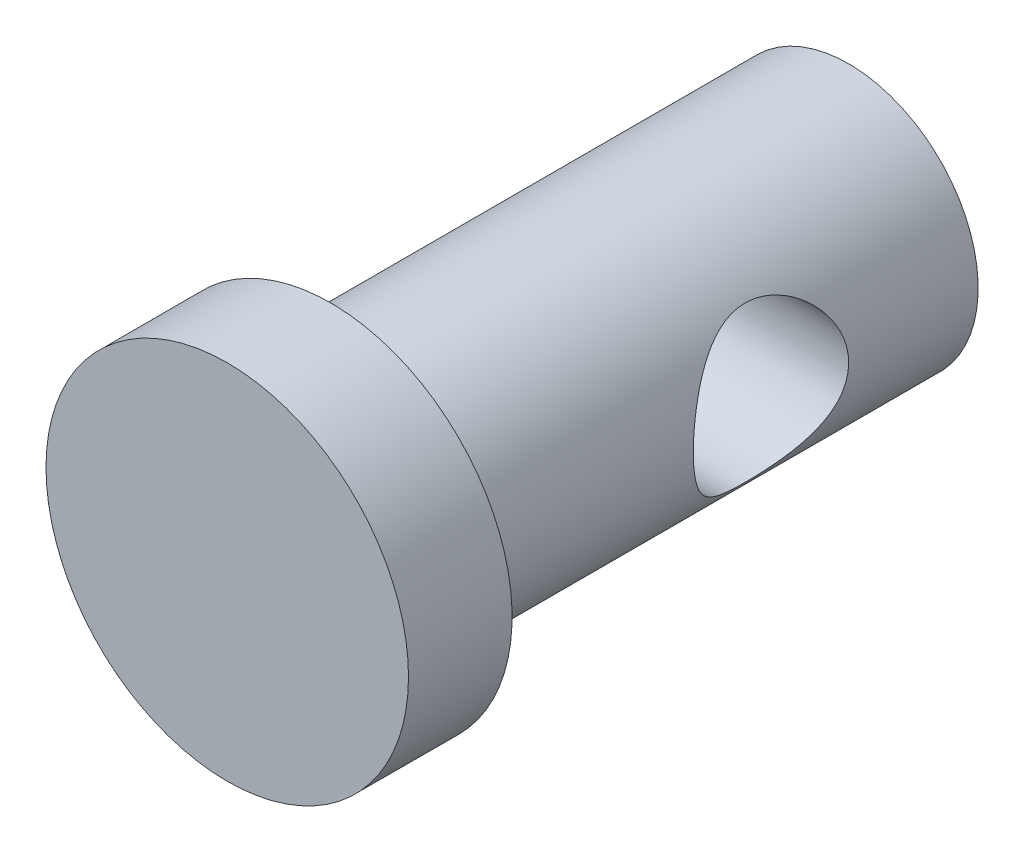
from build123d import *

# Parameters (mm, degrees)
SKETCH1_R           = 17.5
BOSS_EXTRUDE1_DEPTH = 60
CHAMFER1_SIZE       = 1
SKETCH2_R           = 7.5
CUT_EXTRUDE1_DEPTH  = 30
SKETCH3_OUTSIDE_W   = 52.556
SKETCH3_OUTSIDE_H   = 52.556
SKETCH3_OUTSIDE_R   = 12.5
CUT_EXTRUDE2_DEPTH  = 50


with BuildPart() as part:
    # Sketch1 → Boss-Extrude1 (new body)
    with BuildSketch(Plane.XY):
        Circle(SKETCH1_R)
    extrude(amount=BOSS_EXTRUDE1_DEPTH)

    # Chamfer1
    chamfer1_edges = [part.edges().sort_by_distance(p)[0] for p in [
        (-17.5, 0, 0),
    ]]
    chamfer(chamfer1_edges, length=CHAMFER1_SIZE)

    # Sketch2 → Cut-Extrude1 (cut, symmetric)
    with BuildSketch(Plane(origin=(0, 0, 0), x_dir=(0, 0, -1), z_dir=(1, 0, 0))):
        with Locations(Location((-20, 0, 0), (0, 0, 180))):
            Circle(SKETCH2_R)
    extrude(amount=CUT_EXTRUDE1_DEPTH, both=True, mode=Mode.SUBTRACT)

    # Sketch3 outside → Cut-Extrude2 (cut)
    with BuildSketch(Plane(origin=(0, 0, 0), x_dir=(-1, 0, 0), z_dir=(0, 0, -1))):
        Rectangle(SKETCH3_OUTSIDE_W, SKETCH3_OUTSIDE_H)
        Circle(SKETCH3_OUTSIDE_R, mode=Mode.SUBTRACT)
    extrude(amount=-CUT_EXTRUDE2_DEPTH, mode=Mode.SUBTRACT)


solid = part.part
